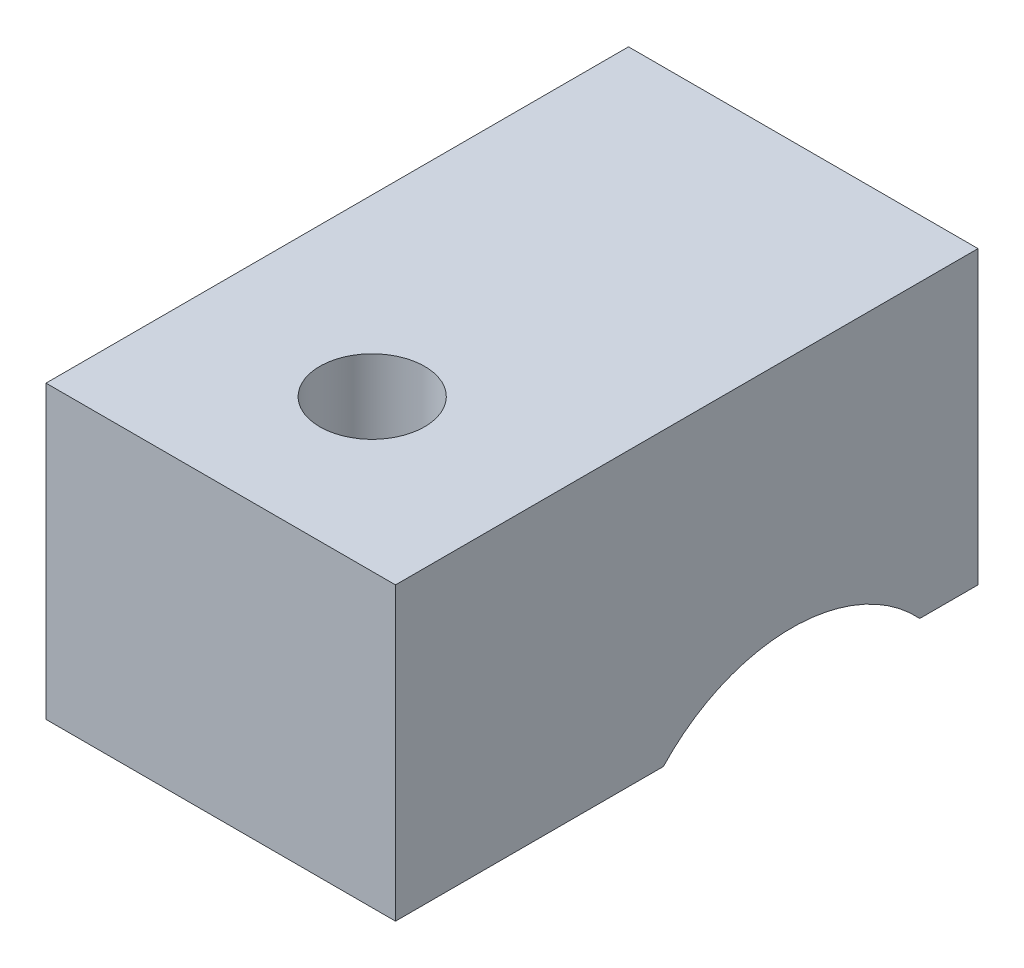
SolidWorks part; units mm, degrees
ref_plane "Front Plane" through (0, 0, 0) normal (0, 0, 1) x (1, 0, 0)
ref_plane "Top Plane" through (0, 0, 0) normal (0, 1, 0) x (1, 0, 0)
ref_plane "Right Plane" through (0, 0, 0) normal (1, 0, 0) x (0, 0, -1)
sketch "Sketch1" plane through (0, 0, 0) normal (0, 0, 1) x (1, 0, 0)
  line L1 (0, 0) -> (30, 0)
  line L2 (0, 0) -> (0, 25)
  line L3 (0, 25) -> (30, 25)
  line L4 (30, 0) -> (30, 25)
  dimension "D1" = 25
  dimension "D2" = 30
extrude "Boss-Extrude1" add sketch "Sketch1" along normal blind 50
sketch "Sketch2" plane through (30, 30, 0) normal (-1, 0, 0) x (0, -1, 0)
  line L4 (0, 5) -> (30, 5) construction
  line L5 (0, 27) -> (30, 27) construction
  line L7 (30, 50) -> (30, 0) construction
  line L8 (30, 27) -> (30, 5)
  line L9 (30, 0) -> (5, 0) construction
  line L10 (30, 50) -> (5, 50) construction
  arc A0 (30, 27) -> (30, 5) centre (40.198, 16) ccw
  dimension "D1" = 30
  dimension "D2" = 5
  dimension "D3" = 23
extrude "Cut-Extrude1" cut sketch "Sketch2" along normal blind 95
hole_wizard "M10x1.0 Tapped Hole1" positions "Sketch4" profile "Sketch3" tap size "M10x1.0" standard "GB" end condition through all
sketch "Sketch4" plane through (0, 25, 0) normal (0, 1, 0) x (-1, 0, 0)
  line L0 (-30, 50) -> (0, 50) construction
  line L1 (0, 50) -> (0, 0) construction
  point P0 (-15, 37)
  dimension "D1" = 13
  dimension "D2" = 15
cosmetic thread "Cosmetic Thread1" parameters "D2"=10
sketch "Sketch3" plane through (15, 25, 37) normal (1, 0, 0) x (0, 0, 1)
  line L0 (0, 0) -> (0, 25)
  line L1 (0, 25) -> (4.5, 25)
  line L2 (4.5, 25) -> (4.5, 0)
  line L5 (4.5, 0) -> (0, 0)
  line L11 (0, -6.35) -> (0, 107.95) construction
  dimension "通孔螺纹孔钻头直径" = 9
  dimension "通孔螺纹孔钻头深度" = 25
